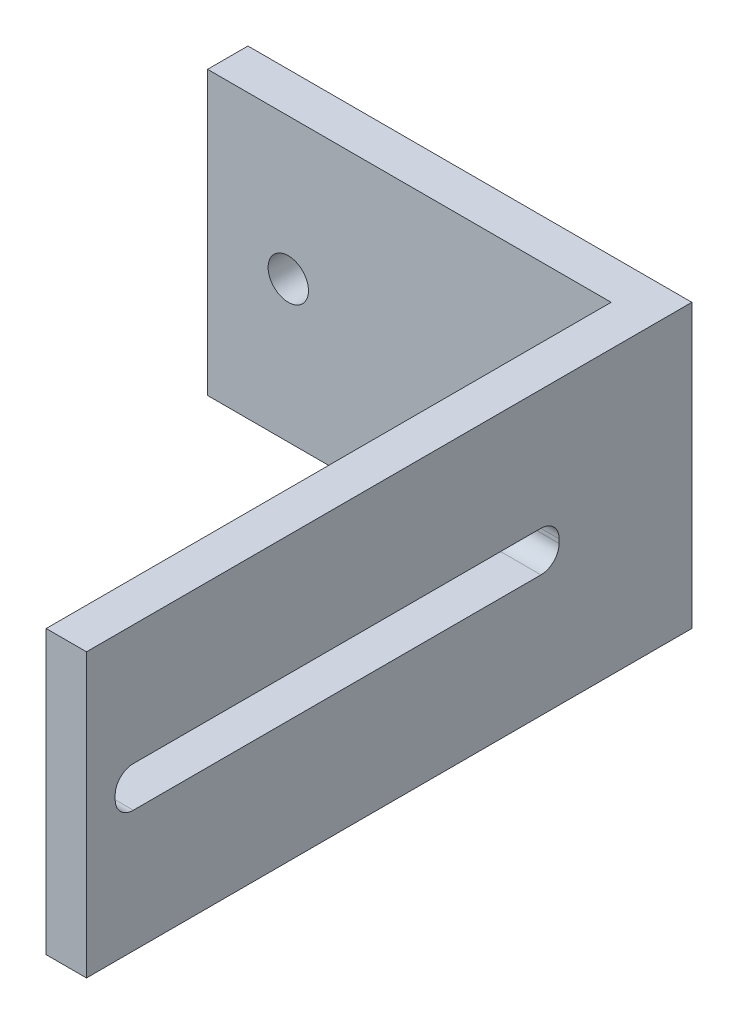
SolidWorks part; units mm, degrees
material "PVC Rigid"
ref_plane "Front Plane" through (0, 0, 0) normal (0, 0, 1) x (1, 0, 0)
ref_plane "Top Plane" through (0, 0, 0) normal (0, 1, 0) x (1, 0, 0)
ref_plane "Right Plane" through (0, 0, 0) normal (1, 0, 0) x (0, 0, -1)
sketch "Sketch1" plane through (0, 0, 0) normal (0, 0, 1) x (1, 0, 0)
  line L1 (50, -35) -> (-50, -35)
  line L2 (50, -35) -> (50, 35)
  line L3 (50, 35) -> (-50, 35)
  line L4 (-50, -35) -> (-50, 35)
  line L5 (50, -35) -> (-50, 35) construction
  line L6 (50, 35) -> (-50, -35) construction
  point P0 (0, 0)
  dimension "D1" = 70
  dimension "D2" = 100
extrude "Boss-Extrude1" add sketch "Sketch1" along normal blind 10
sketch "Sketch2" plane through (0, 0, 10) normal (0, 0, 1) x (1, 0, 0)
  line L0 (50, -35) -> (50, 35) construction
  line L1 (-50, 35) -> (-50, -35) construction
  circle A0 centre (-30, 0) radius 5
  circle A1 centre (30, 0) radius 5
  dimension "D1" = 10
  dimension "D2" = 10
  dimension "D3" = 20
  dimension "D4" = 20
extrude "Cut-Extrude1" cut sketch "Sketch2" against normal blind 10
sketch "Sketch3" plane through (50, 0, 0) normal (1, 0, 0) x (0, 0, -1)
  line L0 (0, 35) -> (-150, 35)
  line L1 (0, -35) -> (-150, -35)
  line L2 (0, 35) -> (0, -35)
  line L3 (-150, 35) -> (-150, -35)
  dimension "D1" = 150
  dimension "D2" = 150
extrude "Boss-Extrude2" add sketch "Sketch3" along normal blind 10
sketch "Sketch7" plane through (50, 0, 0) normal (-1, 0, 0) x (0, 0, 1)
  line L1 (138.3961, -4.7952) -> (37.3961, -4.7952)
  line L2 (142.8961, -0.2952) -> (142.8961, 0.7048)
  line L3 (138.3961, 5.2048) -> (37.3961, 5.2048)
  line L4 (32.8961, -0.2952) -> (32.8961, 0.7048)
  line L5 (142.8961, -4.7952) -> (32.8961, 5.2048) construction
  line L6 (142.8961, 5.2048) -> (32.8961, -4.7952) construction
  arc A0 (142.8961, 0.7048) -> (138.3961, 5.2048) centre (138.3961, 0.7048) ccw
  arc A1 (138.3961, -4.7952) -> (142.8961, -0.2952) centre (138.3961, -0.2952) ccw
  arc A2 (37.3961, -4.7952) -> (32.8961, -0.2952) centre (37.3961, -0.2952) cw
  arc A3 (37.3961, 5.2048) -> (32.8961, 0.7048) centre (37.3961, 0.7048) ccw
  point P0 (87.8961, 0.2048)
  dimension "D3" = 4.5
  dimension "D1" = 10
  dimension "D2" = 110
extrude "Cut-Extrude2" cut sketch "Sketch7" against normal blind 50
